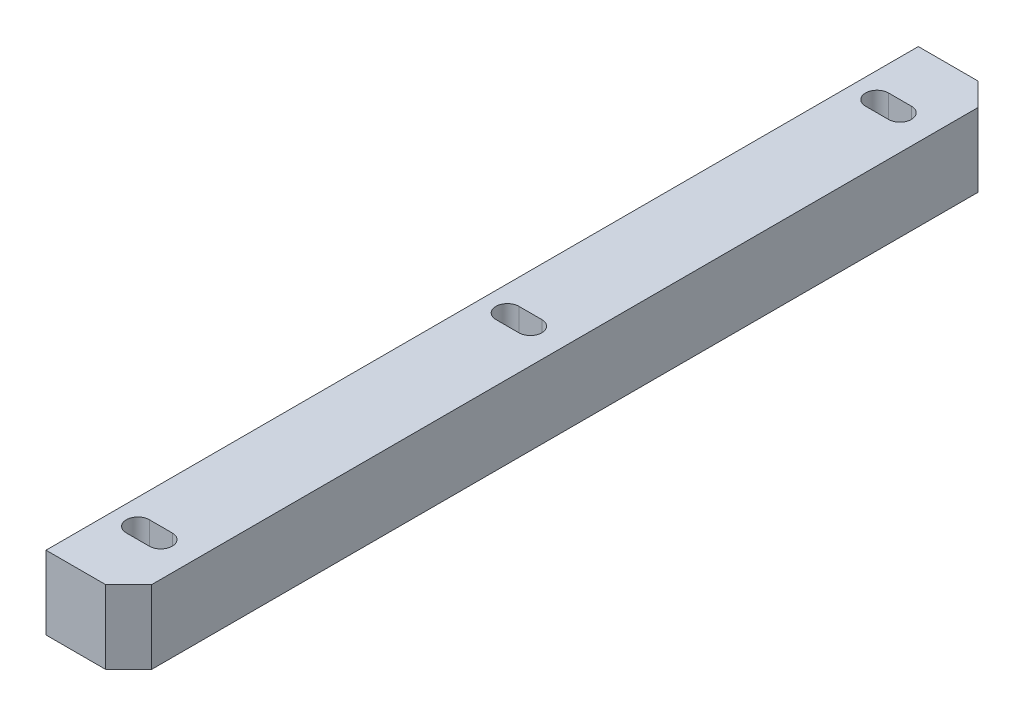
from build123d import *

# Parameters (mm, degrees)
SKETCH_1_W          = 18
SKETCH_1_H          = 16
EXTRUDE_1_DEPTH     = 95
CHAMFER_1_SIZE      = 5
CUT_EXTRUDE_1_REACH = 100.005


with BuildPart() as part:
    # 草图1 → 凸台-拉伸1 (new, symmetric)
    with BuildSketch(Plane.XY):
        with Locations((9, 8)):
            Rectangle(SKETCH_1_W, SKETCH_1_H)
    extrude(amount=EXTRUDE_1_DEPTH, both=True)

    # 倒角1
    chamfer_1_edges = [part.edges().sort_by_distance(p)[0] for p in [
        (18, 8, -95),
        (18, 8, 95),
    ]]
    chamfer(chamfer_1_edges, length=CHAMFER_1_SIZE)

    # 草图2 → 切除-拉伸1 (cut, up to next)
    with BuildSketch(Plane.XZ, mode=Mode.PRIVATE) as cut_extrude_1_sk1:
        with BuildLine():
            Line((5.5, 83), (10.5, 83))
            ThreePointArc((10.5, 83), (13, 80.5), (10.5, 78))
            Line((10.5, 78), (5.5, 78))
            ThreePointArc((5.5, 78), (3, 80.5), (5.5, 83))
        make_face()
    cut_extrude_1_tool1 = extrude(cut_extrude_1_sk1.sketch, amount=-CUT_EXTRUDE_1_REACH, mode=Mode.PRIVATE) & part.part
    # 草图2 → 切除-拉伸1 (cut, up to next)
    with BuildSketch(Plane.XZ, mode=Mode.PRIVATE) as cut_extrude_1_sk2:
        with BuildLine():
            Line((5.5, 2.5), (10.5, 2.5))
            ThreePointArc((10.5, 2.5), (13, 0), (10.5, -2.5))
            Line((10.5, -2.5), (5.5, -2.5))
            ThreePointArc((5.5, -2.5), (3, 0), (5.5, 2.5))
        make_face()
    cut_extrude_1_tool2 = extrude(cut_extrude_1_sk2.sketch, amount=-CUT_EXTRUDE_1_REACH, mode=Mode.PRIVATE) & part.part
    # 草图2 → 切除-拉伸1 (cut, up to next)
    with BuildSketch(Plane.XZ, mode=Mode.PRIVATE) as cut_extrude_1_sk3:
        with BuildLine():
            Line((5.5, -83), (10.5, -83))
            ThreePointArc((10.5, -83), (13, -80.5), (10.5, -78))
            Line((10.5, -78), (5.5, -78))
            ThreePointArc((5.5, -78), (3, -80.5), (5.5, -83))
        make_face()
    cut_extrude_1_tool3 = extrude(cut_extrude_1_sk3.sketch, amount=-CUT_EXTRUDE_1_REACH, mode=Mode.PRIVATE) & part.part
    add(cut_extrude_1_tool1.solids().sort_by_distance((8, 0, 80.5))[0], mode=Mode.SUBTRACT)
    add(cut_extrude_1_tool2.solids().sort_by_distance((8, 0, 0))[0], mode=Mode.SUBTRACT)
    add(cut_extrude_1_tool3.solids().sort_by_distance((8, 0, -80.5))[0], mode=Mode.SUBTRACT)


solid = part.part
